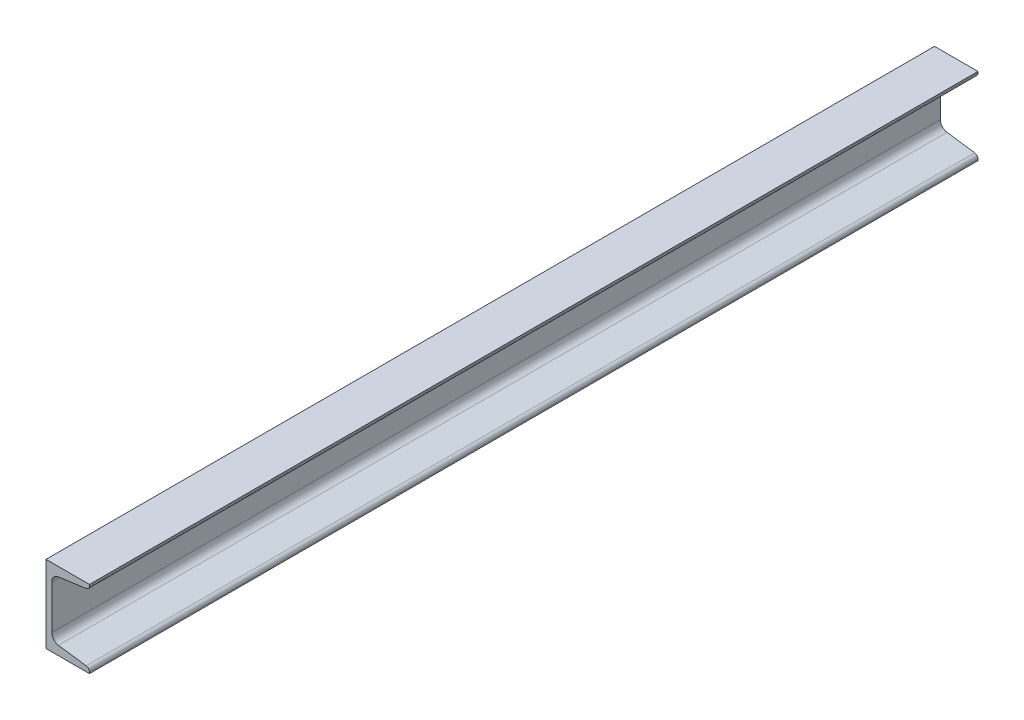
SolidWorks part; units mm, degrees
material "1023 碳钢板 (SS)"
ref_plane "Front Plane" through (0, 0, 0) normal (0, 0, 1) x (1, 0, 0)
ref_plane "Top Plane" through (0, 0, 0) normal (0, 1, 0) x (1, 0, 0)
ref_plane "Right Plane" through (0, 0, 0) normal (1, 0, 0) x (0, 0, -1)
sketch "Sketch1" plane through (0, 0, 0) normal (0, 0, 1) x (1, 0, 0)
  line L0 (0, 0) -> (-45, 0)
  line L1 (-45, 0) -> (-45, -80)
  line L2 (-45, -80) -> (0, -80)
  line L3 (0, -80) -> (0, -78.6393)
  line L4 (-3.4433, -74.6782) -> (-32.1134, -70.6489)
  line L5 (-39, -62.7268) -> (-39, -17.2732)
  line L6 (-32.1134, -9.3511) -> (-3.4433, -5.3218)
  line L7 (0, -1.3607) -> (0, 0)
  line L8 (-22.5, -72) -> (-22.5, -80) construction
  arc A0 (-39, -17.2732) -> (-32.1134, -9.3511) centre (-31, -17.2732) cw
  arc A1 (-32.1134, -70.6489) -> (-39, -62.7268) centre (-31, -62.7268) cw
  arc A2 (-3.4433, -5.3218) -> (0, -1.3607) centre (-4, -1.3607) ccw
  arc A3 (0, -78.6393) -> (-3.4433, -74.6782) centre (-4, -78.6393) ccw
  dimension "D8" = 8
  dimension "D9" = 4
  dimension "D1" = 80
  dimension "D2" = 45
  dimension "D3" = 6
  dimension "D4" = 22.5
  dimension "D5" = 8
  dimension "D6" = 8
  dimension "D7" = 8
extrude "Boss-Extrude1" add sketch "Sketch1" along normal blind 920 contours L7 L0 L1 L2 L3 A3 L4 A1 L5 A0 L6 A2
